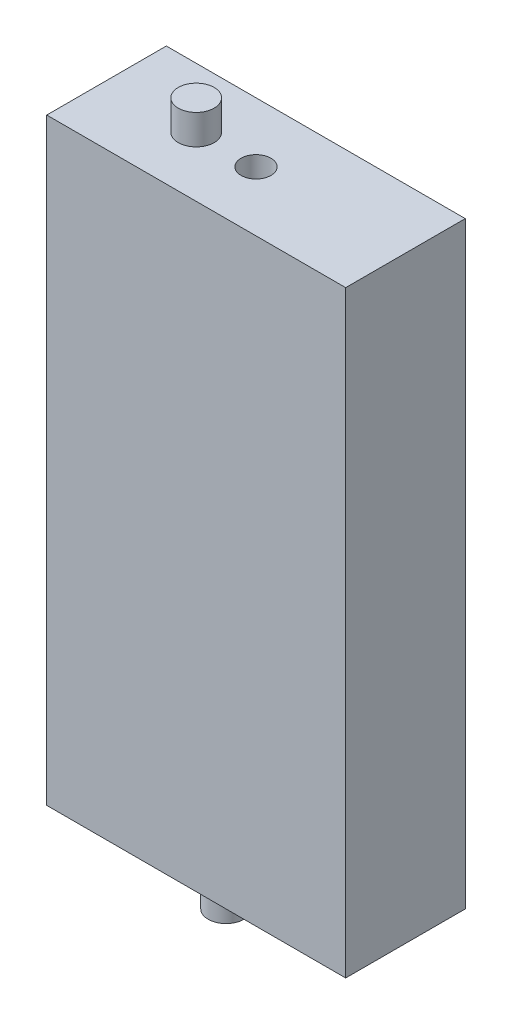
from build123d import *

# Parameters (mm, degrees)
SKETCH1_W             = 50
SKETCH1_H             = 20
BOSS_EXTRUDE1_DEPTH   = 100
SKETCH2_R             = 3
BOSS_EXTRUDE2_DEPTH   = 5
M6_TAPPED_HOLE1_D     = 5
M6_TAPPED_HOLE1_DEPTH = 15
M6_TAPPED_HOLE1_TIP   = 1.502151548
SKETCH5_W             = 20
SKETCH5_H             = 30
BOSS_EXTRUDE3_DEPTH   = 120
M3_TAPPED_HOLE1_D     = 2.5
M3_TAPPED_HOLE1_DEPTH = 7.5
M3_TAPPED_HOLE1_TIP   = 0.751075774
SKETCH8_W             = 147.482871738
SKETCH8_H             = 30
CUT_EXTRUDE1_DEPTH    = 163.249807396
SKETCH9_R             = 3
BOSS_EXTRUDE4_DEPTH   = 5
M6_TAPPED_HOLE2_D     = 5
M6_TAPPED_HOLE2_DEPTH = 15
M6_TAPPED_HOLE2_TIP   = 1.502151548


with BuildPart() as part:
    # Sketch1 → Boss-Extrude1 (new body)
    with BuildSketch(Plane(origin=(0, 0, 0), x_dir=(1, 0, 0), z_dir=(0, 1, 0))):
        Rectangle(SKETCH1_W, SKETCH1_H)
    extrude(amount=BOSS_EXTRUDE1_DEPTH)

    # Sketch2 → Boss-Extrude2 (add)
    with BuildSketch(Plane.XZ):
        with Locations(Location((0, 5, 0), (0, 0, 270))):
            Circle(SKETCH2_R)
    extrude(amount=BOSS_EXTRUDE2_DEPTH)

    # M6 Tapped Hole1
    with Locations(Plane(origin=(0, 0, 0), x_dir=(-1, 0, 0), z_dir=(0, -1, 0))):
        with Locations((0, 5)):
            Hole(M6_TAPPED_HOLE1_D / 2, depth=M6_TAPPED_HOLE1_DEPTH)
            with Locations((0, 0, -(M6_TAPPED_HOLE1_DEPTH + M6_TAPPED_HOLE1_TIP / 2))):  # 118° drill point
                Cone(0, M6_TAPPED_HOLE1_D / 2, M6_TAPPED_HOLE1_TIP, mode=Mode.SUBTRACT)

    # Sketch5 → Boss-Extrude3 (add)
    with BuildSketch(Plane(origin=(25, 0, 0), x_dir=(0, 0, -1), z_dir=(1, 0, 0))):
        with Locations((0, 115)):
            Rectangle(SKETCH5_W, SKETCH5_H)
    extrude(amount=-BOSS_EXTRUDE3_DEPTH)

    # M3 Tapped Hole1
    with Locations(Plane.XY.offset(10)):
        with Locations((-63.4, 108), (-59.4, 112), (-67.4, 105)):
            Hole(M3_TAPPED_HOLE1_D / 2, depth=M3_TAPPED_HOLE1_DEPTH)
            with Locations((0, 0, -(M3_TAPPED_HOLE1_DEPTH + M3_TAPPED_HOLE1_TIP / 2))):  # 118° drill point
                Cone(0, M3_TAPPED_HOLE1_D / 2, M3_TAPPED_HOLE1_TIP, mode=Mode.SUBTRACT)

    # Sketch8 → Cut-Extrude1 (cut, through all)
    with BuildSketch(Plane.XY.offset(10)):
        with Locations((-48.741435869, 115)):
            Rectangle(SKETCH8_W, SKETCH8_H)
    extrude(amount=-CUT_EXTRUDE1_DEPTH, mode=Mode.SUBTRACT)

    # Sketch9 → Boss-Extrude4 (add)
    with BuildSketch(Plane(origin=(0, 100, 0), x_dir=(1, 0, 0), z_dir=(0, 1, 0))):
        with Locations((-10, 0)):
            Circle(SKETCH9_R)
    extrude(amount=BOSS_EXTRUDE4_DEPTH)

    # M6 Tapped Hole2
    with Locations(Plane(origin=(0, 100, 0), x_dir=(1, 0, 0), z_dir=(0, 1, 0))):
        with Locations((0, 0)):
            Hole(M6_TAPPED_HOLE2_D / 2, depth=M6_TAPPED_HOLE2_DEPTH)
            with Locations((0, 0, -(M6_TAPPED_HOLE2_DEPTH + M6_TAPPED_HOLE2_TIP / 2))):  # 118° drill point
                Cone(0, M6_TAPPED_HOLE2_D / 2, M6_TAPPED_HOLE2_TIP, mode=Mode.SUBTRACT)


solid = part.part
